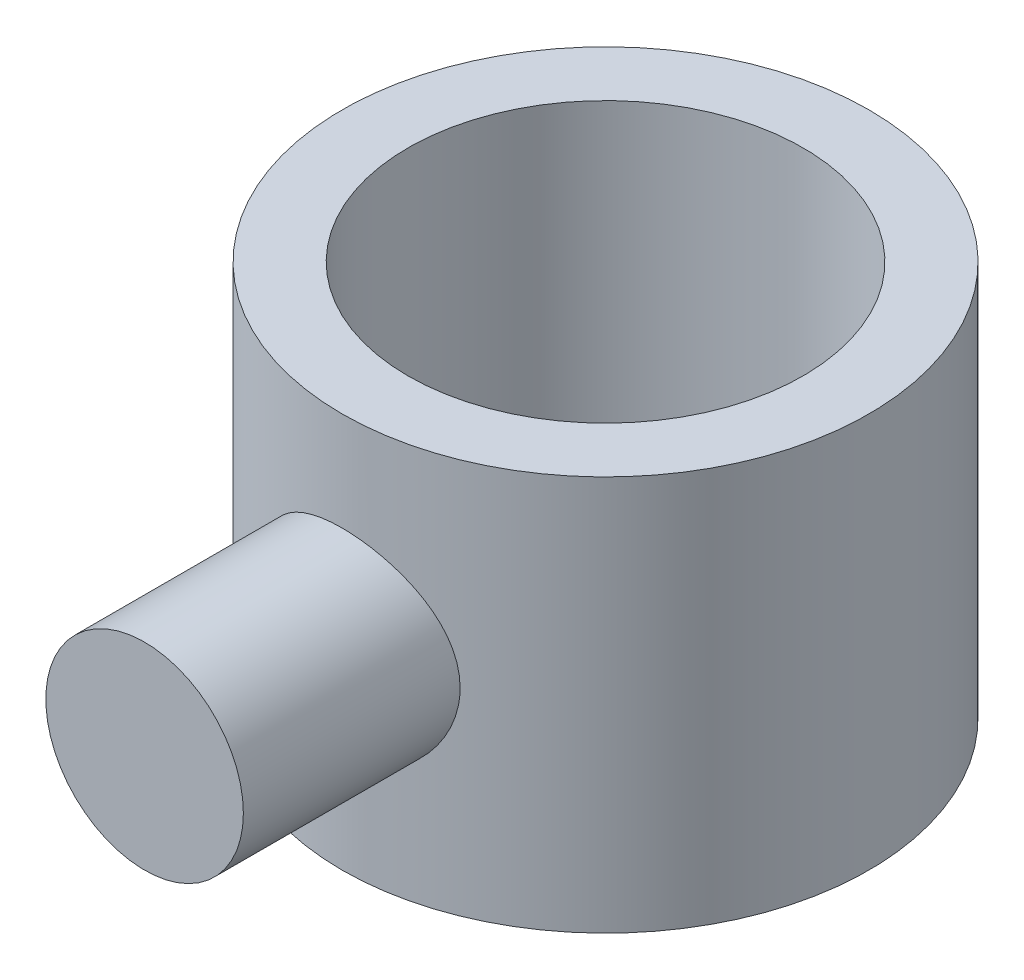
from build123d import *

# Parameters (mm, degrees)
SKETCH1_R                = 4
SKETCH1_R_2              = 3
BOSS_EXTRUDE1_DEPTH      = 6
BOSS_EXTRUDE2_REACH      = 15.153
BOSS_EXTRUDE2_END_RADIUS = 4
SKETCH2_R                = 1.5


with BuildPart() as part:
    # Sketch1 → Boss-Extrude1 (new body)
    with BuildSketch(Plane(origin=(0, 0, 0), x_dir=(1, 0, 0), z_dir=(0, 1, 0))):
        with Locations(Location((0, 0, 0), (0, 0, 270))):
            Circle(SKETCH1_R)
        with Locations(Location((0, 0, 0), (0, 0, 270))):
            Circle(SKETCH1_R_2, mode=Mode.SUBTRACT)
    extrude(amount=BOSS_EXTRUDE1_DEPTH)

    # Boss-Extrude2: up to this cylinder (the profile starts outside it)
    boss_extrude2_end = Plane(origin=(0, 3, 0), z_dir=(0, -1, 0)) * Cylinder(BOSS_EXTRUDE2_END_RADIUS, 39.306, mode=Mode.PRIVATE)
    # Sketch2 → Boss-Extrude2 (add, up to the surface)
    with BuildSketch(Plane.XY.offset(7), mode=Mode.PRIVATE) as boss_extrude2_sk1:
        with Locations((0, 3)):
            Circle(SKETCH2_R)
    boss_extrude2_tool1 = extrude(boss_extrude2_sk1.sketch, amount=-BOSS_EXTRUDE2_REACH, mode=Mode.PRIVATE) - boss_extrude2_end
    add(boss_extrude2_tool1.solids().sort_by_distance((0, 3, 7))[0])


solid = part.part
